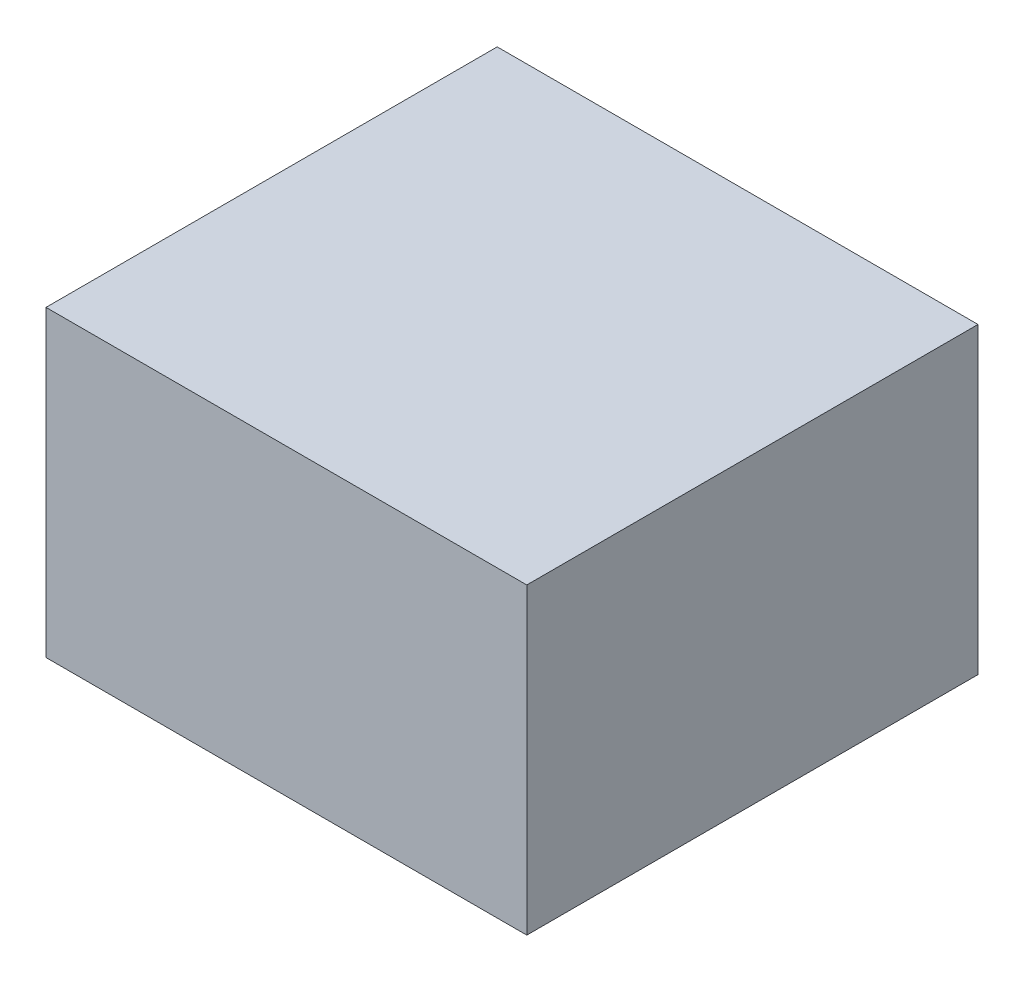
SolidWorks part; units mm, degrees
material "海绵"
ref_plane "Front Plane" through (0, 0, 0) normal (0, 0, 1) x (1, 0, 0)
ref_plane "Top Plane" through (0, 0, 0) normal (0, 1, 0) x (1, 0, 0)
ref_plane "Right Plane" through (0, 0, 0) normal (1, 0, 0) x (0, 0, -1)
sketch "Sketch1" plane through (0, 0, 0) normal (0, 1, 0) x (1, 0, 0)
  line L1 (0, 0) -> (6.5, 0)
  line L2 (0, 0) -> (0, 6.1)
  line L3 (0, 6.1) -> (6.5, 6.1)
  line L4 (6.5, 0) -> (6.5, 6.1)
  dimension "D1" = 6.5
  dimension "D2" = 6.1
extrude "Boss-Extrude1" add sketch "Sketch1" along normal blind 4.1
